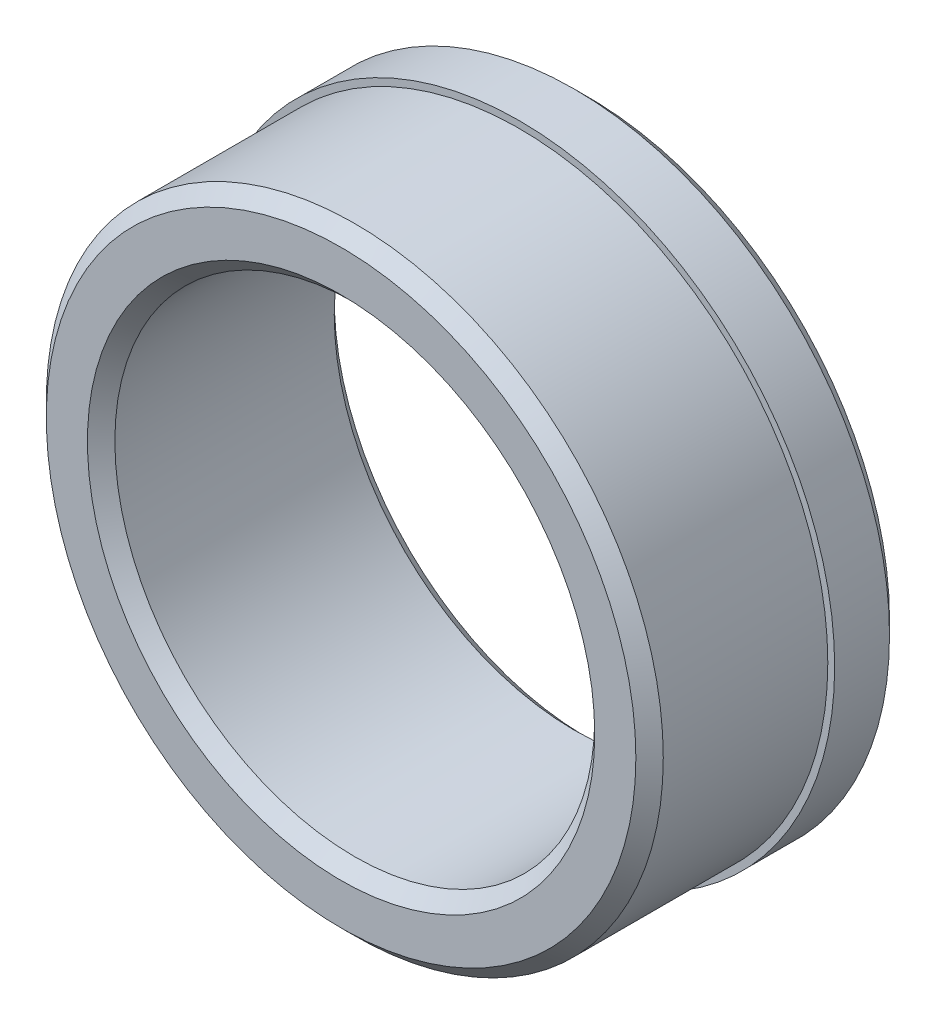
SolidWorks part; units mm, degrees
material "20 steel"
ref_plane "Front Plane" through (0, 0, 0) normal (0, 0, 1) x (1, 0, 0)
ref_plane "Top Plane" through (0, 0, 0) normal (0, 1, 0) x (1, 0, 0)
ref_plane "Right Plane" through (0, 0, 0) normal (1, 0, 0) x (0, 0, -1)
other "Configuration Table"
sketch "Sketch1" plane through (0, 0, 0) normal (1, 0, 0) x (0, 0, -1)
  line L1 (0, 0) -> (26, 0)
  line L2 (0, 0) -> (0, 45)
  line L3 (0, 45) -> (26, 45)
  line L4 (26, 0) -> (26, 45)
  line L5 (26, 0) -> (36, 0)
  line L6 (26, 0) -> (26, 46)
  line L7 (26, 46) -> (36, 46)
  line L8 (36, 0) -> (36, 46)
  line L9 (0, 0) -> (36, 0)
  line L10 (0, 0) -> (0, 35)
  line L11 (0, 35) -> (36, 35)
  line L12 (36, 0) -> (36, 35)
  dimension "D1" = 35
  dimension "D2" = 46
  dimension "D3" = 45
  dimension "D4" = 36
  dimension "D5" = 10
revolve "Revolve1" add sketch "Sketch1" angle 360 about L1
chamfer "Chamfer1" distance 2 angle 45 4 edges at (35, 0, -36) (46, 0, -36) (35, 0, 0) (45, 0, 0)
